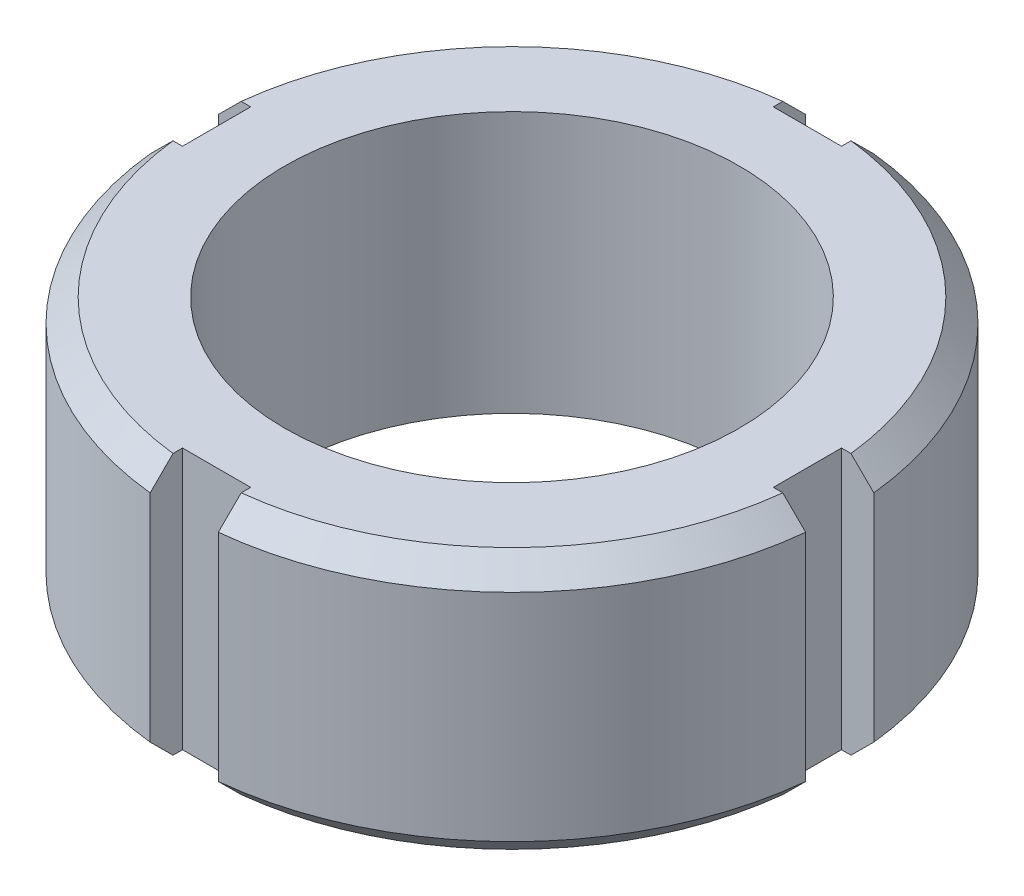
from build123d import *

# Parameters (mm, degrees)
SKETCH1_R           = 29
SKETCH1_R_2         = 20
BOSS_EXTRUDE1_DEPTH = 23
CHAMFER1_SIZE       = 2
SKETCH2_W           = 6
SKETCH2_H           = 12.436847424
CUT_EXTRUDE1_DEPTH  = 48.021271782
CIRPATTERN1_COUNT   = 4


with BuildPart() as part:
    # Sketch1 → Boss-Extrude1 (new body)
    with BuildSketch(Plane(origin=(0, 0, 0), x_dir=(1, 0, 0), z_dir=(0, 1, 0))):
        with Locations(Location((0, 0, 0), (0, 0, 270))):
            Circle(SKETCH1_R)
        with Locations(Location((0, 0, 0), (0, 0, 270))):
            Circle(SKETCH1_R_2, mode=Mode.SUBTRACT)
    extrude(amount=BOSS_EXTRUDE1_DEPTH)

    # Chamfer1
    chamfer1_edges = [part.edges().sort_by_distance(p)[0] for p in [
        (0, 0, -29),
        (0, 23, -29),
    ]]
    chamfer(chamfer1_edges, length=CHAMFER1_SIZE)

    # Sketch2 → Cut-Extrude1 (cut, through all)
    with BuildSketch(Plane(origin=(0, 23, 0), x_dir=(1, 0, 0), z_dir=(0, 1, 0))):
        with Locations((0, 32.218423712)):
            Rectangle(SKETCH2_W, SKETCH2_H)
    cut_extrude1 = extrude(amount=-CUT_EXTRUDE1_DEPTH, mode=Mode.SUBTRACT)

    # CirPattern1: Cut-Extrude1 ×4 about axis
    cirpattern1_axis = Axis((0, 0, 0), (0, 1, 0))
    for i in range(1, CIRPATTERN1_COUNT):
        add(cut_extrude1.rotate(cirpattern1_axis, i * 360 / CIRPATTERN1_COUNT), mode=Mode.SUBTRACT)


solid = part.part
